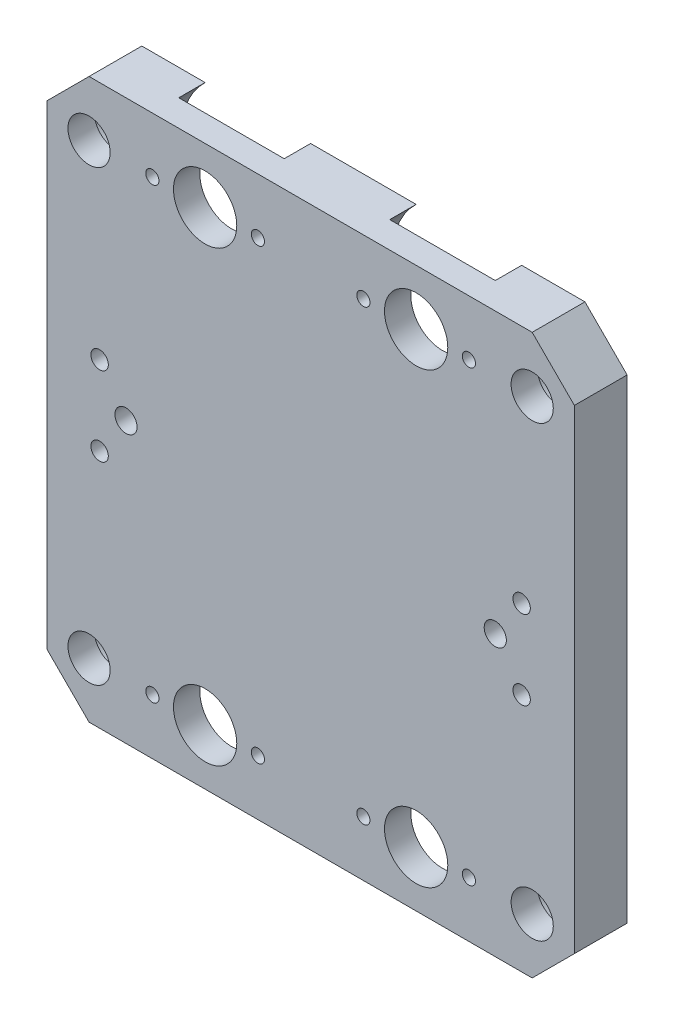
from build123d import *

# Parameters (mm, degrees)
SKETCH_1_W                   = 100
SKETCH_1_H                   = 106
EXTRUDE_1_DEPTH              = 5
HOLE_WIZARD_M5_1_D           = 4.2
CHAMFER_1_SIZE               = 8
HOLE_WIZARD_M4_1_D           = 3.3
SKETCH_10_R                  = 6
EXTRUDE1_DEPTH               = 74.545904033
M3_TAPPED_HOLE1_D            = 2.5
SKETCH3_R                    = 14.5
EXTRUDE2_DEPTH               = 5
F_8_0_8_DIAMETER_HOLE1_D     = 8
F_8_0_8_DIAMETER_HOLE1_DEPTH = 24
F_8_0_8_DIAMETER_HOLE1_TIP   = 2.403442476
SKETCH6_R                    = 6.5
EXTRUDE3_DEPTH               = 5


with BuildPart() as part:
    # 草图1 → 凸台-拉伸1 (new, symmetric)
    with BuildSketch(Plane.XY):
        Rectangle(SKETCH_1_W, SKETCH_1_H)
    extrude(amount=EXTRUDE_1_DEPTH, both=True)

    # M5 螺纹孔1 (through all)
    with Locations(Plane.XY.offset(5)):
        with Locations((-35, 0), (35, 0)):
            Hole(HOLE_WIZARD_M5_1_D / 2)

    # 倒角1
    chamfer_1_edges = [part.edges().sort_by_distance(p)[0] for p in [
        (50, -53, 0),
        (-50, -53, 0),
        (-50, 53, 0),
        (50, 53, 0),
    ]]
    chamfer(chamfer_1_edges, length=CHAMFER_1_SIZE)

    # M4 螺纹孔1 (through all)
    with Locations(Plane.XY.offset(5)):
        with Locations((-40, -7.5), (-40, 7.5)):
            hole_wizard_m4_1 = Hole(HOLE_WIZARD_M4_1_D / 2)

    # 镜向2: M4 螺纹孔1 across plane
    add(hole_wizard_m4_1.mirror(Plane(origin=(0, 0, 0), x_dir=(0, 0, 1), z_dir=(1, 0, 0))), mode=Mode.SUBTRACT)

    # 草图10 → Extrude1 (cut, through all)
    with BuildSketch(Plane.XY.offset(5)):
        with Locations((-20, 42.5)):
            Circle(SKETCH_10_R)
        with Locations((-20, -42.5)):
            Circle(SKETCH_10_R)
        with Locations((20, -42.5)):
            Circle(SKETCH_10_R)
        with Locations((20, 42.5)):
            Circle(SKETCH_10_R)
    extrude(amount=-EXTRUDE1_DEPTH, mode=Mode.SUBTRACT)

    # M3 Tapped Hole1 (through all)
    with Locations(Plane.XY.offset(5)):
        with Locations((10, -42.5), (30, -42.5), (-10, -42.5), (-30, -42.5), (-10, 42.5), (-30, 42.5), (10, 42.5), (30, 42.5)):
            Hole(M3_TAPPED_HOLE1_D / 2)

    # Sketch3 → Extrude2 (cut)
    with BuildSketch(Plane.XY.offset(-5)):
        with Locations((-20, 42.5)):
            Circle(SKETCH3_R)
        with Locations((-20, -42.5)):
            Circle(SKETCH3_R)
        with Locations((20, -42.5)):
            Circle(SKETCH3_R)
        with Locations((20, 42.5)):
            Circle(SKETCH3_R)
    extrude(amount=EXTRUDE2_DEPTH, mode=Mode.SUBTRACT)

    # Ø8.0 (8) Diameter Hole1
    with Locations(Plane.XY.offset(5)):
        with Locations((-42, 42.5), (42, 42.5), (42, -42.5), (-42, -42.5)):
            Hole(F_8_0_8_DIAMETER_HOLE1_D / 2, depth=F_8_0_8_DIAMETER_HOLE1_DEPTH)
            with Locations((0, 0, -(F_8_0_8_DIAMETER_HOLE1_DEPTH + F_8_0_8_DIAMETER_HOLE1_TIP / 2))):  # 118° drill point
                Cone(0, F_8_0_8_DIAMETER_HOLE1_D / 2, F_8_0_8_DIAMETER_HOLE1_TIP, mode=Mode.SUBTRACT)

    # Sketch6 → Extrude3 (cut)
    with BuildSketch(Plane(origin=(0, 0, -5), x_dir=(-1, 0, 0), z_dir=(0, 0, -1))):
        with Locations((42, -42.5)):
            Circle(SKETCH6_R)
        with Locations((-42, -42.5)):
            Circle(SKETCH6_R)
        with Locations((42, 42.5)):
            Circle(SKETCH6_R)
        with Locations((-42, 42.5)):
            Circle(SKETCH6_R)
    extrude(amount=-EXTRUDE3_DEPTH, mode=Mode.SUBTRACT)


solid = part.part
